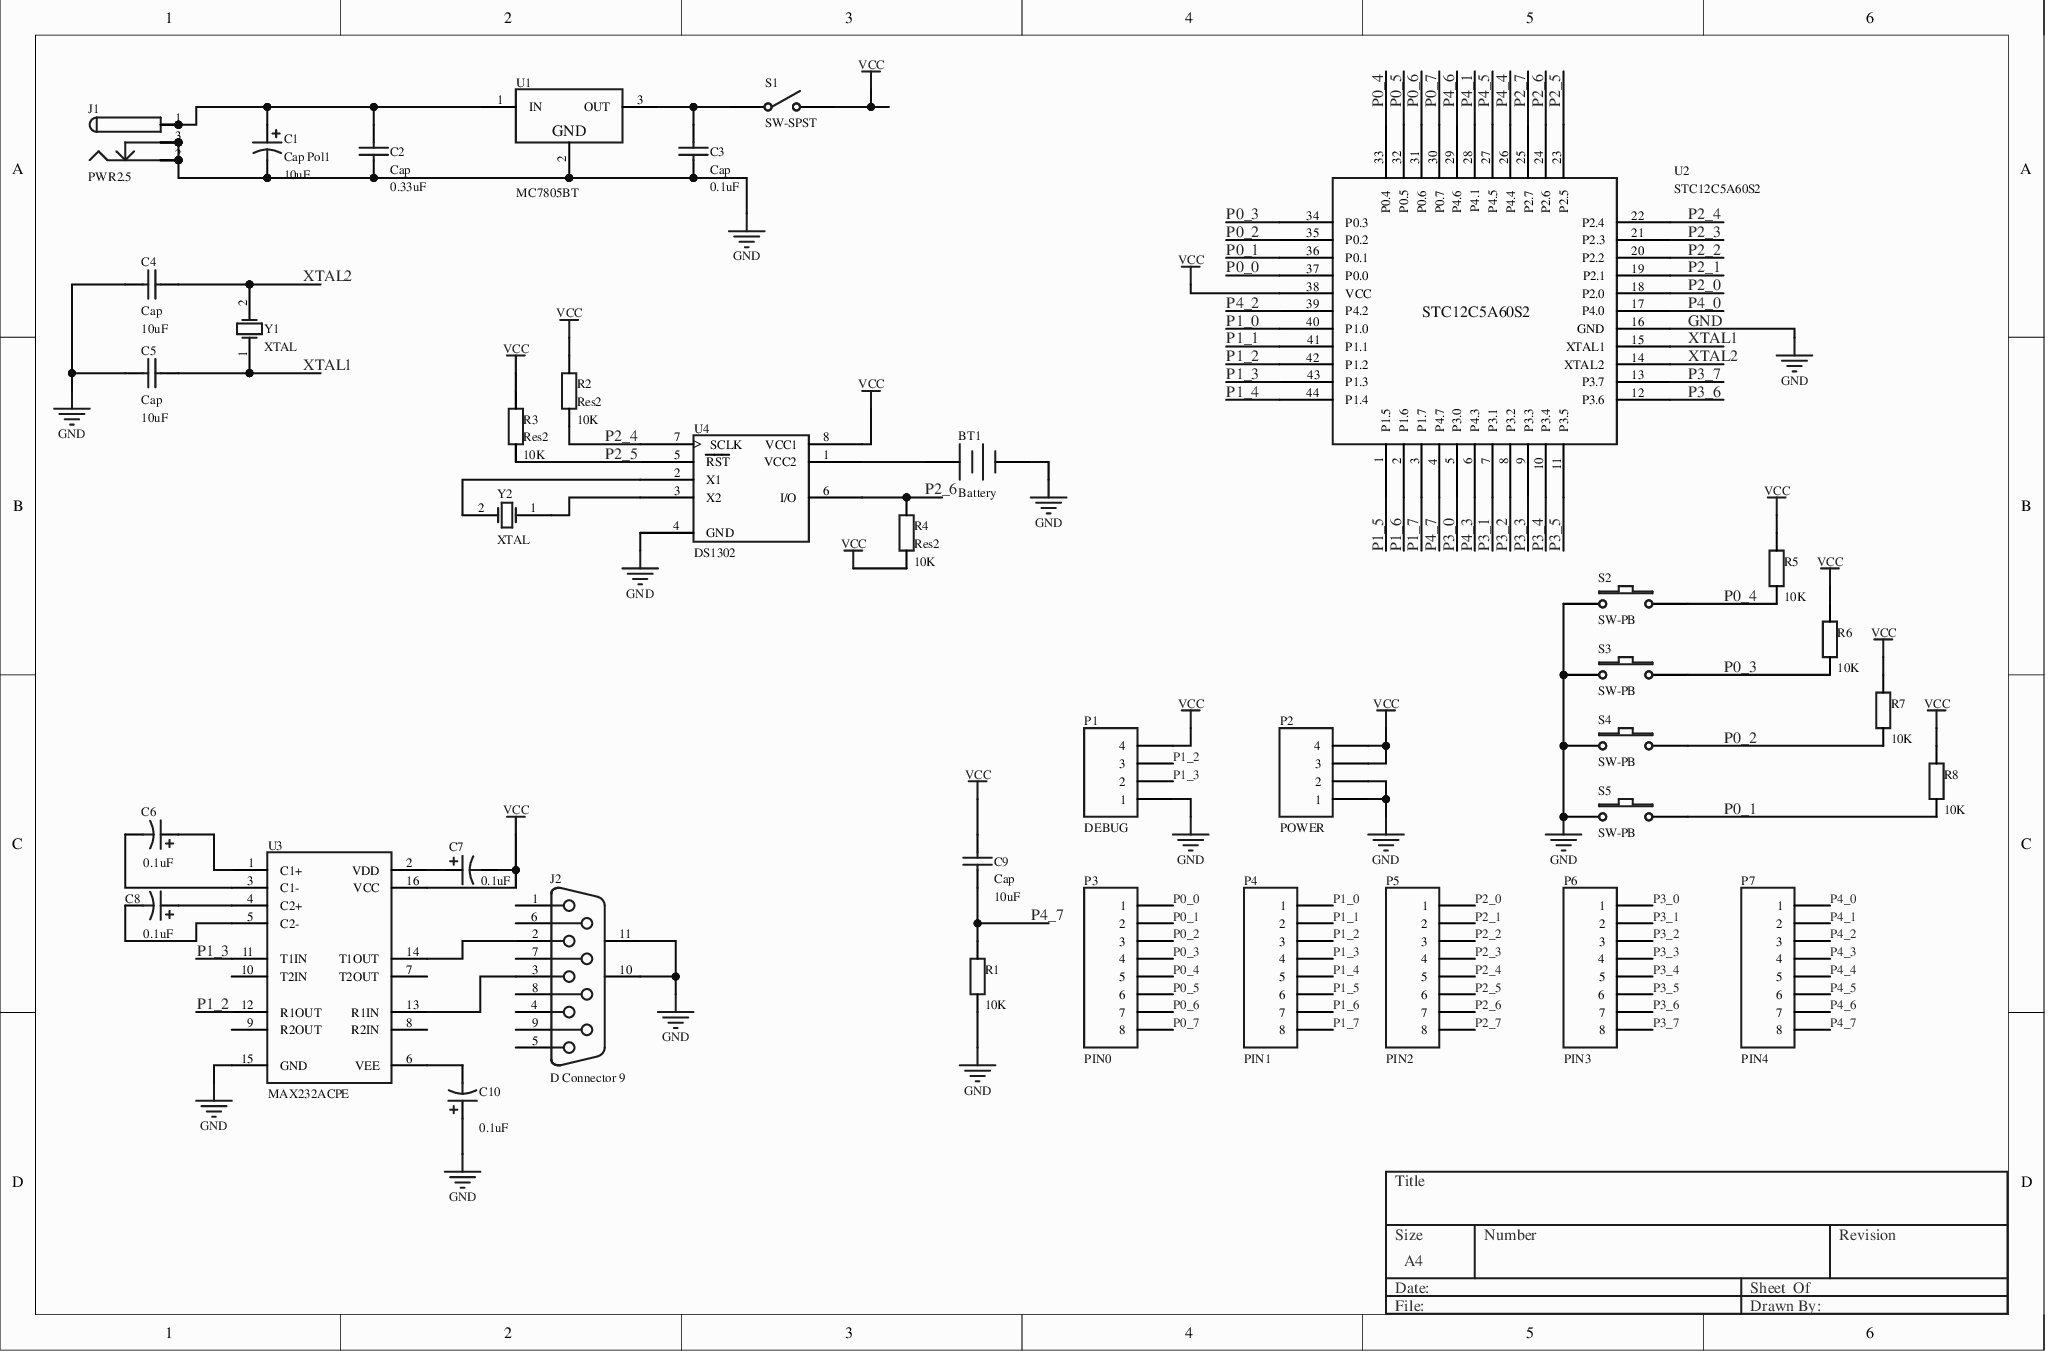
[diagram p0: MISC50994-3.schdoc]
# Altium project MISC50994-2.PrjPcb
1 sheet, 39 parts. Net scope: global (net labels, ports and power ports of the same name join across sheets).
Board file: MISC50994.pcbdoc

## Sheet MISC50994-3.schdoc
size 292 x 193 mm

### Parts
BT1  Battery  [BAT-2]
C1  Cap Pol1  value 10uF  [RB2.54-5.08]
C2  Cap  value 0.33uF  [RAD-0.3]
C3  Cap  value 0.1uF  [C0805]
C4  Cap  value 10uF  [C0805]
C5  Cap  value 10uF  [C0805]
C6  value 0.1uF  [RB2.54-5.08]  (hidden comment: Cap Pol1)
C7  value 0.1uF  [RB2.54-5.08]  (hidden comment: Cap Pol1)
C8  value 0.1uF  [RB2.54-5.08]  (hidden comment: Cap Pol1)
C9  Cap  value 10uF  [C0805]
C10  value 0.1uF  [RB2.54-5.08]  (hidden comment: Cap Pol1)
J1  PWR2.5  [KLD-0202]
J2  D Connector 9  [DSUB1.385-2H9]
P1  DEBUG  [HDR1X4]
P2  POWER  [HDR1X4]
P3  PIN0  [HDR1X8]
P4  PIN1  [HDR1X8]
P5  PIN2  [HDR1X8]
P6  PIN3  [HDR1X8]
P7  PIN4  [HDR1X8]
R1  value 10K  [6-0805_L]  (hidden comment: Res2)
R2  Res2  value 10K  [6-0805_L]
R3  Res2  value 10K  [6-0805_L]
R4  Res2  value 10K  [6-0805_L]
R5  value 10K  [6-0805_L]  (hidden comment: Res2)
R6  value 10K  [6-0805_L]  (hidden comment: Res2)
R7  value 10K  [6-0805_L]  (hidden comment: Res2)
R8  value 10K  [6-0805_L]  (hidden comment: Res2)
S1  SW-SPST  [SPST-2]
S2  SW-PB  [SPST-2]
S3  SW-PB  [SPST-2]
S4  SW-PB  [SPST-2]
S5  SW-PB  [SPST-2]
U1  MC7805BT  [221A-04]
U2  STC12C5A60S2  [TQFP-44]
U3  MAX232ACPE  [PE16A]
U4  DS1302  [DIP-8]
Y1  XTAL  [R38]
Y2  XTAL  [R38]

### Nets
GND: BT1.2(-) C1.2 C2.1 C3.1 C4.2 C5.2 C10.1 J1.2 J1.2A J1.2B J1.3 J1.3A J1.3B J2.10(MH1) J2.11(MH2) P1.1 P2.1 P2.2 R1.1 S2.1 S3.1 S4.1 S5.1 U1.2(GND) U2.16(GND) U3.15(GND) U4.4(GND)
VCC: C7.2 C9.2 P1.4 P2.3 P2.4 R2.2 R3.2 R4.1 R5.2 R6.2 R7.2 R8.2 S1.2(NO) U2.38(VCC) U3.16(VCC) U4.8(VCC1)
P0_0: P3.1 U2.37(P0.0)
P0_1: P3.2 R8.1 S5.2 U2.36(P0.1)
P0_2: P3.3 R7.1 S4.2 U2.35(P0.2)
P0_3: P3.4 R6.1 S3.2 U2.34(P0.3)
P0_4: P3.5 R5.1 S2.2 U2.33(P0.4)
P0_5: P3.6 U2.32(P0.5)
P0_6: P3.7 U2.31(P0.6)
P0_7: P3.8 U2.30(P0.7)
P1_0: P4.1 U2.40(P1.0)
P1_1: P4.2 U2.41(P1.1)
P1_2: P1.3 P4.3 U2.42(P1.2) U3.12(R1OUT)
P1_3: P1.2 P4.4 U2.43(P1.3) U3.11(T1IN)
P1_4: P4.5 U2.44(P1.4)
P1_5: P4.6 U2.1(P1.5)
P1_6: P4.7 U2.2(P1.6)
P1_7: P4.8 U2.3(P1.7)
P2_0: P5.1 U2.18(P2.0)
P2_1: P5.2 U2.19(P2.1)
P2_2: P5.3 U2.20(P2.2)
P2_3: P5.4 U2.21(P2.3)
P2_4: P5.5 R2.1 U2.22(P2.4) U4.7(SCLK)
P2_5: P5.6 R3.1 U2.23(P2.5) U4.5(~{RST})
P2_6: P5.7 R4.2 U2.24(P2.6) U4.6(I/O)
P2_7: P5.8 U2.25(P2.7)
P3_0: P6.1 U2.5(P3.0)
P3_1: P6.2 U2.7(P3.1)
P3_2: P6.3 U2.8(P3.2)
P3_3: P6.4 U2.9(P3.3)
P3_4: P6.5 U2.10(P3.4)
P3_5: P6.6 U2.11(P3.5)
P3_6: P6.7 U2.12(P3.6)
P3_7: P6.8 U2.13(P3.7)
P4_0: P7.1 U2.17(P4.0)
P4_1: P7.2 U2.28(P4.1)
P4_2: P7.3 U2.39(P4.2)
P4_3: P7.4 U2.6(P4.3)
P4_4: P7.5 U2.26(P4.4)
P4_5: P7.6 U2.27(P4.5)
P4_6: P7.7 U2.29(P4.6)
P4_7: C9.1 P7.8 R1.2 U2.4(P4.7)
XTAL1: C5.1 U2.15(XTAL1) Y1.1(OSC1)
XTAL2: C4.1 U2.14(XTAL2) Y1.2(OSC2)
NetBT1_1: BT1.1(+) U4.1(VCC2)
NetC1_1: C1.1 C2.2 J1.1 J1.1A J1.1B U1.1(IN)
NetC3_2: C3.2 S1.1(COMMON) U1.3(OUT)
NetC6_1: C6.1 U3.1(C1+)
NetC6_2: C6.2 U3.3(C1-)
NetC7_1: C7.1 U3.2(VDD)
NetC8_1: C8.1 U3.4(C2+)
NetC8_2: C8.2 U3.5(C2-)
NetC10_2: C10.2 U3.6(VEE)
NetJ2_2: J2.2 U3.14(T1OUT)
NetJ2_3: J2.3 U3.13(R1IN)
NetU4_2: U4.2(X1) Y2.2(OSC2)
NetU4_3: U4.3(X2) Y2.1(OSC1)

Not connected (* = marked no-connect by the designer): J2 1 4 5 6 7 8 9; U3 7(T2OUT)* 8(R2IN)* 9(R2OUT)* 10(T2IN)*

### Notes on the sheet
- Title
- File:
- Date:
- Size
- A4
- Number
- Drawn By:
- Sheet
- Of
- Revision

### Library data of the parts
BT1 = Battery: Multicell Battery; UniqueId: c9182c8b26c7f8f5; AddInBom: yes; Origin Footprint: BAT-2; Device: Battery; Symbol: Battery; Design Item ID: Battery; Library Name: Miscellaneous Devices; Published: 24-Mar-1999; LatestRevisionDate: 17-Jul-2002; LatestRevisionNote: Re-released for DXP Platform.; PackageReference: BAT-2; PackageDescription: Battery; 2 Leads; FootprintName: BAT-2; ConvertToPcb: yes; Publisher: Altium Limited
C1 = Cap Pol1: Polarized Capacitor (Radial); Origin Footprint 2: RB7.6-15; Origin Footprint 3: RB-.2/.5; UniqueId: b4693cfd16d534cd; AddInBom: yes; Origin Footprint 1: RB2.54-5.08; Device: Cap Pol1; Symbol: Cap Pol1; Design Item ID: Cap Pol1; Library Name: Miscellaneous Devices; Published: 8-Jun-2000; LatestRevisionDate: 17-Jul-2002; LatestRevisionNote: Re-released for DXP Platform.; PackageReference: RB7.6-15; PackageDescription: Polarized Capacitor (Radial); 2 Leads; FootprintName: RB2.54-5.08; Origin Footprint 4: RB2.54-5.08; ConvertToPcb: yes; Publisher: Altium Limited
C2 = Cap: Capacitor; UniqueId: a2c5d49bc5dde298; AddInBom: yes; Origin Footprint: RAD-0.3; Device: Cap; Symbol: Cap; Design Item ID: Cap; Library Name: Miscellaneous Devices; Published: 8-Jun-2000; LatestRevisionDate: 17-Jul-2002; LatestRevisionNote: Re-released for DXP Platform.; PackageReference: RAD-0.3; PackageDescription: Radial Cap, Thru-Hole; 2 Leads; 0.3 in Pin Spacing; FootprintName: RAD-0.3; ConvertToPcb: yes; Publisher: Altium Limited
C3 = Cap: Capacitor; Origin Footprint 2: RAD-0.3; UniqueId: cc82bf2c2e22e605; AddInBom: yes; Origin Footprint 1: C0805; Device: Cap; Symbol: Cap; Design Item ID: Cap; Library Name: Miscellaneous Devices; Published: 8-Jun-2000; LatestRevisionDate: 17-Jul-2002; LatestRevisionNote: Re-released for DXP Platform.; PackageReference: RAD-0.3; PackageDescription: Radial Cap, Thru-Hole; 2 Leads; 0.3 in Pin Spacing; FootprintName: C0805; ConvertToPcb: yes; Publisher: Altium Limited
C4 = Cap: Capacitor; Origin Footprint 2: RAD-0.3; UniqueId: 3a68d3ddabf48558; AddInBom: yes; Origin Footprint 1: C0805; Device: Cap; Symbol: Cap; Design Item ID: Cap; Library Name: Miscellaneous Devices; Published: 8-Jun-2000; LatestRevisionDate: 17-Jul-2002; LatestRevisionNote: Re-released for DXP Platform.; PackageReference: RAD-0.3; PackageDescription: Radial Cap, Thru-Hole; 2 Leads; 0.3 in Pin Spacing; FootprintName: C0805; ConvertToPcb: yes; Publisher: Altium Limited
C5 = Cap: Capacitor; Origin Footprint 2: RAD-0.3; UniqueId: ddba3c46cf8b8e66; AddInBom: yes; Origin Footprint 1: C0805; Device: Cap; Symbol: Cap; Design Item ID: Cap; Library Name: Miscellaneous Devices; Published: 8-Jun-2000; LatestRevisionDate: 17-Jul-2002; LatestRevisionNote: Re-released for DXP Platform.; PackageReference: RAD-0.3; PackageDescription: Radial Cap, Thru-Hole; 2 Leads; 0.3 in Pin Spacing; FootprintName: C0805; ConvertToPcb: yes; Publisher: Altium Limited
C6 = Cap Pol1: Polarized Capacitor (Radial); Origin Footprint 2: RB7.6-15; Origin Footprint 3: RB-.2/.5; UniqueId: ab4a8fe24fad9fe4; AddInBom: yes; Origin Footprint 1: RB2.54-5.08; Device: Cap Pol1; Symbol: Cap Pol1; Design Item ID: Cap Pol1; Library Name: Miscellaneous Devices; Published: 8-Jun-2000; LatestRevisionDate: 17-Jul-2002; LatestRevisionNote: Re-released for DXP Platform.; PackageReference: RB7.6-15; PackageDescription: Polarized Capacitor (Radial); 2 Leads; FootprintName: RB2.54-5.08; Origin Footprint 4: RB2.54-5.08; ConvertToPcb: yes; Publisher: Altium Limited
C7 = Cap Pol1: Polarized Capacitor (Radial); Origin Footprint 2: RB7.6-15; Origin Footprint 3: RB-.2/.5; UniqueId: 48d2dd422533522c; AddInBom: yes; Origin Footprint 1: RB2.54-5.08; Device: Cap Pol1; Symbol: Cap Pol1; Design Item ID: Cap Pol1; Library Name: Miscellaneous Devices; Published: 8-Jun-2000; LatestRevisionDate: 17-Jul-2002; LatestRevisionNote: Re-released for DXP Platform.; PackageReference: RB7.6-15; PackageDescription: Polarized Capacitor (Radial); 2 Leads; FootprintName: RB2.54-5.08; Origin Footprint 4: RB2.54-5.08; ConvertToPcb: yes; Publisher: Altium Limited
C8 = Cap Pol1: Polarized Capacitor (Radial); Origin Footprint 2: RB7.6-15; Origin Footprint 3: RB-.2/.5; UniqueId: 80f3708378e3d903; AddInBom: yes; Origin Footprint 1: RB2.54-5.08; Device: Cap Pol1; Symbol: Cap Pol1; Design Item ID: Cap Pol1; Library Name: Miscellaneous Devices; Published: 8-Jun-2000; LatestRevisionDate: 17-Jul-2002; LatestRevisionNote: Re-released for DXP Platform.; PackageReference: RB7.6-15; PackageDescription: Polarized Capacitor (Radial); 2 Leads; Origin Footprint 4: RB2.54-5.08; FootprintName: RB2.54-5.08; ConvertToPcb: yes; Publisher: Altium Limited
C9 = Cap: Capacitor; Origin Footprint 2: RAD-0.3; UniqueId: 7ddfd2f632a8b17d; AddInBom: yes; Origin Footprint 1: C0805; Device: Cap; Symbol: Cap; Design Item ID: Cap; Library Name: Miscellaneous Devices; Published: 8-Jun-2000; LatestRevisionDate: 17-Jul-2002; LatestRevisionNote: Re-released for DXP Platform.; PackageReference: RAD-0.3; PackageDescription: Radial Cap, Thru-Hole; 2 Leads; 0.3 in Pin Spacing; FootprintName: C0805; ConvertToPcb: yes; Publisher: Altium Limited
C10 = Cap Pol1: Polarized Capacitor (Radial); Origin Footprint 2: RB7.6-15; Origin Footprint 3: RB-.2/.5; UniqueId: 3e75135af30e0f04; AddInBom: yes; Origin Footprint 1: RB2.54-5.08; Device: Cap Pol1; Symbol: Cap Pol1; Design Item ID: Cap Pol1; Library Name: Miscellaneous Devices; Published: 8-Jun-2000; LatestRevisionDate: 17-Jul-2002; LatestRevisionNote: Re-released for DXP Platform.; PackageReference: RB7.6-15; PackageDescription: Polarized Capacitor (Radial); 2 Leads; FootprintName: RB2.54-5.08; Origin Footprint 4: RB2.54-5.08; ConvertToPcb: yes; Publisher: Altium Limited
J1 = PWR2.5: Low Voltage Power Supply Connector; UniqueId: 51bfc0e5166a1c40; AddInBom: yes; Origin Footprint: KLD-0202; Device: PWR2.5; Symbol: PWR2.5; Design Item ID: PWR2.5; Library Name: Miscellaneous Connectors; Published: 17-Dec-2003; DatasheetDocument: 09-May-2002; ComponentLink1Description: Manufacturer Link; FootprintName: KLD-0202; ConvertToPcb: yes; Publisher: Altium Limited
J2 = D Connector 9: Receptacle Assembly, 9 Position, Right Angle; PackageDocument: O; Positions: 9; UniqueId: 1fb9863844ab5169; AddInBom: yes; Origin Footprint: DSUB1.385-2H9; Device: D Connector 9; Symbol: D Connector 9; Design Item ID: D Connector 9; Library Name: Miscellaneous Connectors; Published: 15-Jun-2001; LatestRevisionDate: 17-Jul-2002; LatestRevisionNote: Re-released for DXP Platform.; DatasheetDocument: 1-Sep-1999; PackageReference: 788750; Orientation: Right Angle; Gender: Receptacle; FootprintName: DSUB1.385-2H9; ConvertToPcb: yes; Publisher: Altium Limited
P1 = DEBUG: Header, 4-Pin; Symbol: Header 4; UniqueId: c39ee3c861a7b382; AddInBom: yes; Origin Footprint: HDR1X4; Device: DEBUG; Design Item ID: Header 4; Library Name: Miscellaneous Connectors; LatestRevisionDate: 17-Jul-2002; LatestRevisionNote: Re-released for DXP Platform.; FootprintName: HDR1X4; ConvertToPcb: yes; Publisher: Altium Limited
P2 = POWER: Header, 4-Pin; Symbol: Header 4; UniqueId: 16cbebb8866e1842; AddInBom: yes; Origin Footprint: HDR1X4; Device: POWER; Design Item ID: Header 4; Library Name: Miscellaneous Connectors; LatestRevisionDate: 17-Jul-2002; LatestRevisionNote: Re-released for DXP Platform.; FootprintName: HDR1X4; ConvertToPcb: yes; Publisher: Altium Limited
P3 = PIN0: Header, 8-Pin; Symbol: Header 8; UniqueId: 1bc31e334497ec54; AddInBom: yes; Origin Footprint: HDR1X8; Device: PIN0; Design Item ID: Header 8; Library Name: Miscellaneous Connectors; LatestRevisionDate: 17-Jul-2002; LatestRevisionNote: Re-released for DXP Platform.; FootprintName: HDR1X8; ConvertToPcb: yes; Publisher: Altium Limited
P4 = PIN1: Header, 8-Pin; Symbol: Header 8; UniqueId: 6a809a8f8408ed49; AddInBom: yes; Origin Footprint: HDR1X8; Device: PIN1; Design Item ID: Header 8; Library Name: Miscellaneous Connectors; LatestRevisionDate: 17-Jul-2002; LatestRevisionNote: Re-released for DXP Platform.; FootprintName: HDR1X8; ConvertToPcb: yes; Publisher: Altium Limited
P5 = PIN2: Header, 8-Pin; Symbol: Header 8; UniqueId: a30bd92ff87464e3; AddInBom: yes; Origin Footprint: HDR1X8; Device: PIN2; Design Item ID: Header 8; Library Name: Miscellaneous Connectors; LatestRevisionDate: 17-Jul-2002; LatestRevisionNote: Re-released for DXP Platform.; FootprintName: HDR1X8; ConvertToPcb: yes; Publisher: Altium Limited
P6 = PIN3: Header, 8-Pin; Symbol: Header 8; UniqueId: 2d4d75c2fcc000cd; AddInBom: yes; Origin Footprint: HDR1X8; Device: PIN3; Design Item ID: Header 8; Library Name: Miscellaneous Connectors; LatestRevisionDate: 17-Jul-2002; LatestRevisionNote: Re-released for DXP Platform.; FootprintName: HDR1X8; ConvertToPcb: yes; Publisher: Altium Limited
P7 = PIN4: Header, 8-Pin; Symbol: Header 8; UniqueId: f2444bf4b29cd8fb; AddInBom: yes; Origin Footprint: HDR1X8; Device: PIN4; Design Item ID: Header 8; Library Name: Miscellaneous Connectors; LatestRevisionDate: 17-Jul-2002; LatestRevisionNote: Re-released for DXP Platform.; FootprintName: HDR1X8; ConvertToPcb: yes; Publisher: Altium Limited
R1 = Res2: Resistor; Origin Footprint 2: AXIAL-0.4; UniqueId: 353b166cc2dee846; AddInBom: yes; Origin Footprint 1: 6-0805_L; Device: Res2; Symbol: Res2; Design Item ID: Res2; Library Name: Miscellaneous Devices; Published: 8-Jun-2000; LatestRevisionDate: 17-Jul-2002; LatestRevisionNote: Re-released for DXP Platform.; PackageReference: AXIAL-0.4; PackageDescription: Axial Device, Thru-Hole; 2 Leads; 0.4 in Pin Spacing; FootprintName: 6-0805_L; ConvertToPcb: yes; Publisher: Altium Limited
R2 = Res2: Resistor; Origin Footprint 2: AXIAL-0.4; UniqueId: 6f63fc6711cfa315; AddInBom: yes; Origin Footprint 1: 6-0805_L; Device: Res2; Symbol: Res2; Design Item ID: Res2; Library Name: Miscellaneous Devices; Published: 8-Jun-2000; LatestRevisionDate: 17-Jul-2002; LatestRevisionNote: Re-released for DXP Platform.; PackageReference: AXIAL-0.4; PackageDescription: Axial Device, Thru-Hole; 2 Leads; 0.4 in Pin Spacing; FootprintName: 6-0805_L; ConvertToPcb: yes; Publisher: Altium Limited
R3 = Res2: Resistor; Origin Footprint 2: AXIAL-0.4; UniqueId: fe89d0632cfce75f; AddInBom: yes; Origin Footprint 1: 6-0805_L; Device: Res2; Symbol: Res2; Design Item ID: Res2; Library Name: Miscellaneous Devices; Published: 8-Jun-2000; LatestRevisionDate: 17-Jul-2002; LatestRevisionNote: Re-released for DXP Platform.; PackageReference: AXIAL-0.4; PackageDescription: Axial Device, Thru-Hole; 2 Leads; 0.4 in Pin Spacing; FootprintName: 6-0805_L; ConvertToPcb: yes; Publisher: Altium Limited
R4 = Res2: Resistor; Origin Footprint 2: AXIAL-0.4; UniqueId: fdc86a4b576d9e98; AddInBom: yes; Origin Footprint 1: 6-0805_L; Device: Res2; Symbol: Res2; Design Item ID: Res2; Library Name: Miscellaneous Devices; Published: 8-Jun-2000; LatestRevisionDate: 17-Jul-2002; LatestRevisionNote: Re-released for DXP Platform.; PackageReference: AXIAL-0.4; PackageDescription: Axial Device, Thru-Hole; 2 Leads; 0.4 in Pin Spacing; FootprintName: 6-0805_L; ConvertToPcb: yes; Publisher: Altium Limited
R5 = Res2: Resistor; Origin Footprint 2: AXIAL-0.4; UniqueId: 9cdd622c9eeecfe7; AddInBom: yes; Origin Footprint 1: 6-0805_L; Device: Res2; Symbol: Res2; Design Item ID: Res2; Library Name: Miscellaneous Devices; Published: 8-Jun-2000; LatestRevisionDate: 17-Jul-2002; LatestRevisionNote: Re-released for DXP Platform.; PackageReference: AXIAL-0.4; PackageDescription: Axial Device, Thru-Hole; 2 Leads; 0.4 in Pin Spacing; FootprintName: 6-0805_L; ConvertToPcb: yes; Publisher: Altium Limited
R6 = Res2: Resistor; Origin Footprint 2: AXIAL-0.4; UniqueId: e06ccd13940482ac; AddInBom: yes; Origin Footprint 1: 6-0805_L; Device: Res2; Symbol: Res2; Design Item ID: Res2; Library Name: Miscellaneous Devices; Published: 8-Jun-2000; LatestRevisionDate: 17-Jul-2002; LatestRevisionNote: Re-released for DXP Platform.; PackageReference: AXIAL-0.4; PackageDescription: Axial Device, Thru-Hole; 2 Leads; 0.4 in Pin Spacing; FootprintName: 6-0805_L; ConvertToPcb: yes; Publisher: Altium Limited
R7 = Res2: Resistor; Origin Footprint 2: AXIAL-0.4; UniqueId: ba2c6d155e7fd301; AddInBom: yes; Origin Footprint 1: 6-0805_L; Device: Res2; Symbol: Res2; Design Item ID: Res2; Library Name: Miscellaneous Devices; Published: 8-Jun-2000; LatestRevisionDate: 17-Jul-2002; LatestRevisionNote: Re-released for DXP Platform.; PackageReference: AXIAL-0.4; PackageDescription: Axial Device, Thru-Hole; 2 Leads; 0.4 in Pin Spacing; FootprintName: 6-0805_L; ConvertToPcb: yes; Publisher: Altium Limited
R8 = Res2: Resistor; Origin Footprint 2: AXIAL-0.4; UniqueId: 86d447fa2a9c8586; AddInBom: yes; Origin Footprint 1: 6-0805_L; Device: Res2; Symbol: Res2; Design Item ID: Res2; Library Name: Miscellaneous Devices; Published: 8-Jun-2000; LatestRevisionDate: 17-Jul-2002; LatestRevisionNote: Re-released for DXP Platform.; PackageReference: AXIAL-0.4; PackageDescription: Axial Device, Thru-Hole; 2 Leads; 0.4 in Pin Spacing; FootprintName: 6-0805_L; ConvertToPcb: yes; Publisher: Altium Limited
S1 = SW-SPST: Single-Pole, Single-Throw Switch; UniqueId: 0ac0bd892f9b1ec0; AddInBom: yes; Origin Footprint: SPST-2; Device: SW-SPST; Symbol: SW-SPST; Design Item ID: SW-SPST; Library Name: Miscellaneous Devices; Published: 24-Mar-1999; LatestRevisionDate: 17-Jul-2002; LatestRevisionNote: Re-released for DXP Platform.; PackageReference: SPST-2; PackageDescription: Switch; 2 Leads; FootprintName: SPST-2; ConvertToPcb: yes; Publisher: Altium Limited
S2 = SW-PB: Switch; UniqueId: 16ca49f37df57620; AddInBom: yes; Origin Footprint: SPST-2; Device: SW-PB; Symbol: SW-PB; Design Item ID: SW-PB; Library Name: Miscellaneous Devices; Published: 24-Mar-1999; LatestRevisionDate: 17-Jul-2002; LatestRevisionNote: Re-released for DXP Platform.; PackageReference: SPST-2; PackageDescription: Switch; 2 Leads; FootprintName: SPST-2; ConvertToPcb: yes; Publisher: Altium Limited
S3 = SW-PB: Switch; UniqueId: b21ed8cc1c3b642b; AddInBom: yes; Origin Footprint: SPST-2; Device: SW-PB; Symbol: SW-PB; Design Item ID: SW-PB; Library Name: Miscellaneous Devices; Published: 24-Mar-1999; LatestRevisionDate: 17-Jul-2002; LatestRevisionNote: Re-released for DXP Platform.; PackageReference: SPST-2; PackageDescription: Switch; 2 Leads; FootprintName: SPST-2; ConvertToPcb: yes; Publisher: Altium Limited
S4 = SW-PB: Switch; UniqueId: b4af5bc4dd85243d; AddInBom: yes; Origin Footprint: SPST-2; Device: SW-PB; Symbol: SW-PB; Design Item ID: SW-PB; Library Name: Miscellaneous Devices; Published: 24-Mar-1999; LatestRevisionDate: 17-Jul-2002; LatestRevisionNote: Re-released for DXP Platform.; PackageReference: SPST-2; PackageDescription: Switch; 2 Leads; FootprintName: SPST-2; ConvertToPcb: yes; Publisher: Altium Limited
S5 = SW-PB: Switch; UniqueId: b2403b9688924408; AddInBom: yes; Origin Footprint: SPST-2; Device: SW-PB; Symbol: SW-PB; Design Item ID: SW-PB; Library Name: Miscellaneous Devices; Published: 24-Mar-1999; LatestRevisionDate: 17-Jul-2002; LatestRevisionNote: Re-released for DXP Platform.; PackageReference: SPST-2; PackageDescription: Switch; 2 Leads; FootprintName: SPST-2; ConvertToPcb: yes; Publisher: Altium Limited
U1 = MC7805BT: 3-Terminal Positive Fixed Voltage Regulator; Note: Pin 2 is electrically connected to TAB; UniqueId: 1bdc0ab44f99f92d; AddInBom: yes; Origin Footprint: 221A-04; Device: MC7805BT; Symbol: MC7805BT; Design Item ID: MC7805BT; Library Name: Motorola Power Mgt Voltage Regulator; Published: 17-Jul-2002; DatasheetVersion: 1988; PackageReference: 221A-04; PackageDescription: TO, Thru-Hole, Vertical, Heatsink Mounted; 3 In-Line Leads; Pitch 2.54 mm; Code_JEDEC: TO-262-AA; ComponentLink1Description: Manufacturer Link; ComponentLink1URL: http://www.onsemi.com/site/products/taxonomy/0,4438,503,00.html; Datasheet: http://www.onsemi.com/pub/Collateral/MC7800-D.PDF; ComponentLink2Description: Datasheet; ComponentLink2URL: http://www.onsemi.com/pub/Collateral/MC7800-D.PDF; FootprintName: 221A-04; ConvertToPcb: yes; Publisher: Altium Limited
U2 = STC12C5A60S2: UniqueId: 48f0ae2437312dae; AddInBom: yes; Origin Footprint: TQFP-44; Device: STC12C5A60S2; Symbol: STC12C5A60S2; Design Item ID: STC12C5A60S2; Library Name: Schlib1; FootprintName: TQFP-44; ConvertToPcb: yes
U3 = MAX232ACPE: +5V Powered, Multi-Channel RS-232 Driver/Receiver; UniqueId: 66797bcd97f4f6c2; AddInBom: yes; Origin Footprint: PE16A; Device: MAX232ACPE; Symbol: MAX232ACPE; Design Item ID: MAX232ACPE; Library Name: Maxim Communication Transceiver; Published: 16-Jan-2001; LatestRevisionDate: 29-May-2009; LatestRevisionNote: Component Body Added.; PackageVersion: 1997; PackageReference: PE16A; PackageDescription: DIP, 16-Pin, Row Spacing 7.62 mm, Pitch 2.54 mm; Code_JEDEC: MS-001-BB; ComponentLink1Description: Manufacturer Link; Datasheet: http://pdfserv.maxim-ic.com/en/ds/MAX220-MAX249.pdf; ComponentLink2Description: Datasheet; ComponentLink2URL: http://pdfserv.maxim-ic.com/en/ds/MAX220-MAX249.pdf; FootprintName: PE16A; ConvertToPcb: yes; Publisher: Altium Limited
U4 = DS1302: UniqueId: bac468049775df37; AddInBom: yes; ModelId: b25ce56d62334bb48ac4eeaf82c54c81; Origin Footprint: DIP-8; Device: DS1302; Symbol: DS1302; Design Item ID: DS1302; Library Name: lixiqing-zlg; FootprintName: DIP-8; ConvertToPcb: yes; ModelName: DIP-8
Y1 = XTAL: Crystal Oscillator; UniqueId: 9790cc8ece124e27; AddInBom: yes; Origin Footprint: R38; Device: XTAL; Symbol: XTAL; Design Item ID: XTAL; Library Name: Miscellaneous Devices; Published: 8-Jun-2000; LatestRevisionDate: 17-Jul-2002; LatestRevisionNote: Re-released for DXP Platform.; PackageReference: R38; PackageDescription: Crystal, Thru-Hole; 2 Leads; Body 3.1 x 8.2 mm (Dia.xH); FootprintName: R38; ConvertToPcb: yes; Publisher: Altium Limited
Y2 = XTAL: Crystal Oscillator; UniqueId: 54aa28710a128dff; AddInBom: yes; Origin Footprint: R38; Device: XTAL; Symbol: XTAL; Design Item ID: XTAL; Library Name: Miscellaneous Devices; Published: 8-Jun-2000; LatestRevisionDate: 17-Jul-2002; LatestRevisionNote: Re-released for DXP Platform.; PackageReference: R38; PackageDescription: Crystal, Thru-Hole; 2 Leads; Body 3.1 x 8.2 mm (Dia.xH); FootprintName: R38; ConvertToPcb: yes; Publisher: Altium Limited